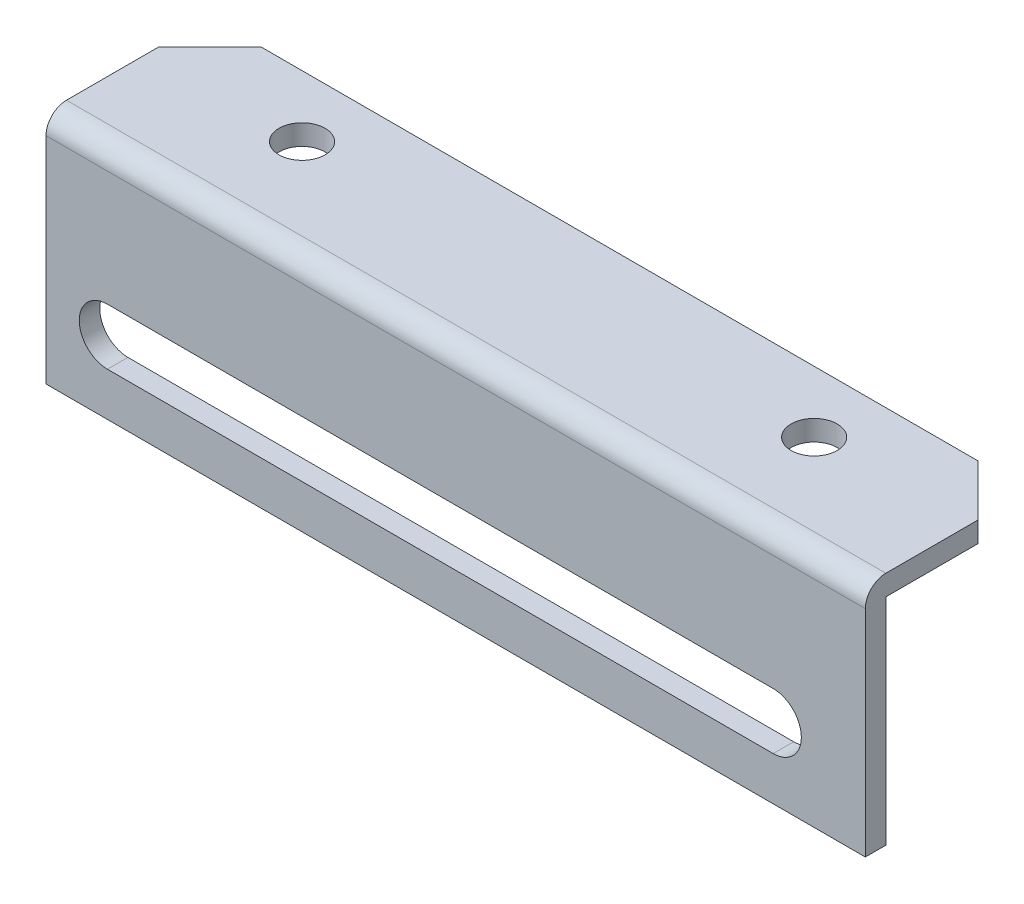
from build123d import *

# Parameters (mm, degrees)
SKETCH_1_W             = 150
SKETCH_1_H             = 25
BOSS_EXTRUDE_1_DEPTH   = 18
SKETCH_2_W             = 16
SKETCH_2_H             = 23
CUT_EXTRUDE_1_DEPTH    = 152.592381075
CUT_EXTRUDE_3_DEPTH    = 79.136099212
F_4_5_4_5_HOLE_1_D     = 4.5
F_4_5_4_5_HOLE_1_DEPTH = 15
F_4_5_4_5_HOLE_1_TIP   = 1.351936393
F_4_5_4_5_HOLE_3_D     = 4.5
F_4_5_4_5_HOLE_3_DEPTH = 15
F_4_5_4_5_HOLE_3_TIP   = 1.351936393
F_4_5_4_5_HOLE_2_D     = 4.5
F_4_5_4_5_HOLE_2_DEPTH = 15
F_4_5_4_5_HOLE_2_TIP   = 1.351936393
CHAMFER_1_SIZE         = 2
FILLET_1_R             = 2
SKETCH_11_W            = 150
SKETCH_11_H            = 2
CUT_EXTRUDE_4_DEPTH    = 10
CHAMFER_4_SIZE         = 5
SKETCH_12_W            = 121.932032981
SKETCH_12_H            = 48.36827262
CUT_EXTRUDE_5_DEPTH    = 78.699742599
CHAMFER_5_SIZE         = 5
SKETCH_13_W            = 80
SKETCH_13_H            = 2
CUT_EXTRUDE_6_DEPTH    = 10


with BuildPart() as part:
    # Sketch 1 → Boss-Extrude 1 (new body)
    with BuildSketch(Plane(origin=(0, 0, 0), x_dir=(-1, 0, 0), z_dir=(0, 0, -1))):
        Rectangle(SKETCH_1_W, SKETCH_1_H)
    extrude(amount=-BOSS_EXTRUDE_1_DEPTH)

    # Sketch 2 → Cut-Extrude 1 (cut, through all)
    with BuildSketch(Plane.ZY.offset(75)):
        with Locations((8, -1)):
            Rectangle(SKETCH_2_W, SKETCH_2_H)
    extrude(amount=-CUT_EXTRUDE_1_DEPTH, mode=Mode.SUBTRACT)

    # Sketch 4 → Cut-Extrude 3 (cut, through all)
    with BuildSketch(Plane.XY.offset(18)):
        with BuildLine():
            Line((-69, -6.25), (-4, -6.25))
            ThreePointArc((-4, -6.25), (-1.25, -3.5), (-4, -0.75))
            Line((-4, -0.75), (-69, -0.75))
            ThreePointArc((-69, -0.75), (-71.75, -3.5), (-69, -6.25))
        make_face()
    extrude(amount=-CUT_EXTRUDE_3_DEPTH, mode=Mode.SUBTRACT)

    # Ø4.5 (4.5) Hole 1
    with Locations(Plane(origin=(0, 12.5, 0), x_dir=(-1, 0, 0), z_dir=(0, 1, 0))):
        with Locations((-60, 8)):
            Hole(F_4_5_4_5_HOLE_1_D / 2, depth=F_4_5_4_5_HOLE_1_DEPTH)
            with Locations((0, 0, -(F_4_5_4_5_HOLE_1_DEPTH + F_4_5_4_5_HOLE_1_TIP / 2))):  # 118° drill point
                Cone(0, F_4_5_4_5_HOLE_1_D / 2, F_4_5_4_5_HOLE_1_TIP, mode=Mode.SUBTRACT)

    # Ø4.5 (4.5) Hole 3
    with Locations(Plane(origin=(0, 12.5, 0), x_dir=(-1, 0, 0), z_dir=(0, 1, 0))):
        with Locations((60, 8)):
            Hole(F_4_5_4_5_HOLE_3_D / 2, depth=F_4_5_4_5_HOLE_3_DEPTH)
            with Locations((0, 0, -(F_4_5_4_5_HOLE_3_DEPTH + F_4_5_4_5_HOLE_3_TIP / 2))):  # 118° drill point
                Cone(0, F_4_5_4_5_HOLE_3_D / 2, F_4_5_4_5_HOLE_3_TIP, mode=Mode.SUBTRACT)

    # Ø4.5 (4.5) Hole 2
    with Locations(Plane(origin=(0, 12.5, 0), x_dir=(-1, 0, 0), z_dir=(0, 1, 0))):
        with Locations((10, 8)):
            Hole(F_4_5_4_5_HOLE_2_D / 2, depth=F_4_5_4_5_HOLE_2_DEPTH)
            with Locations((0, 0, -(F_4_5_4_5_HOLE_2_DEPTH + F_4_5_4_5_HOLE_2_TIP / 2))):  # 118° drill point
                Cone(0, F_4_5_4_5_HOLE_2_D / 2, F_4_5_4_5_HOLE_2_TIP, mode=Mode.SUBTRACT)

    # Chamfer 1
    chamfer_1_edges = [part.edges().sort_by_distance(p)[0] for p in [
        (75, -12.5, 17),
    ]]
    chamfer(chamfer_1_edges, length=CHAMFER_1_SIZE)

    # Fillet 1
    fillet_1_edges = [part.edges().sort_by_distance(p)[0] for p in [
        (0, 12.5, 18),
    ]]
    fillet(fillet_1_edges, radius=FILLET_1_R)

    # Sketch 11 → Cut-Extrude 4 (cut)
    with BuildSketch(Plane(origin=(0, 12.5, 0), x_dir=(1, 0, 0), z_dir=(0, 1, 0))):
        with Locations((0, -1)):
            Rectangle(SKETCH_11_W, SKETCH_11_H)
    extrude(amount=-CUT_EXTRUDE_4_DEPTH, mode=Mode.SUBTRACT)

    # Chamfer 4
    chamfer_4_edges = [part.edges().sort_by_distance(p)[0] for p in [
        (75, 11.5, 2),
        (-75, 11.5, 2),
    ]]
    chamfer(chamfer_4_edges, length=CHAMFER_4_SIZE)

    # Sketch 12 → Cut-Extrude 5 (cut, through all)
    with BuildSketch(Plane(origin=(0, 0, 2), x_dir=(-1, 0, 0), z_dir=(0, 0, -1))):
        with Locations((-65.966016491, 1.254835332)):
            Rectangle(SKETCH_12_W, SKETCH_12_H)
    extrude(amount=-CUT_EXTRUDE_5_DEPTH, mode=Mode.SUBTRACT)

    # Chamfer 5
    chamfer_5_edges = [part.edges().sort_by_distance(p)[0] for p in [
        (5, 11.5, 2),
    ]]
    chamfer(chamfer_5_edges, length=CHAMFER_5_SIZE)

    # Sketch 13 → Cut-Extrude 6 (cut)
    with BuildSketch(Plane(origin=(0, 0, 16), x_dir=(-1, 0, 0), z_dir=(0, 0, -1))):
        with Locations((35, -11.5)):
            Rectangle(SKETCH_13_W, SKETCH_13_H)
    extrude(amount=-CUT_EXTRUDE_6_DEPTH, mode=Mode.SUBTRACT)


solid = part.part
